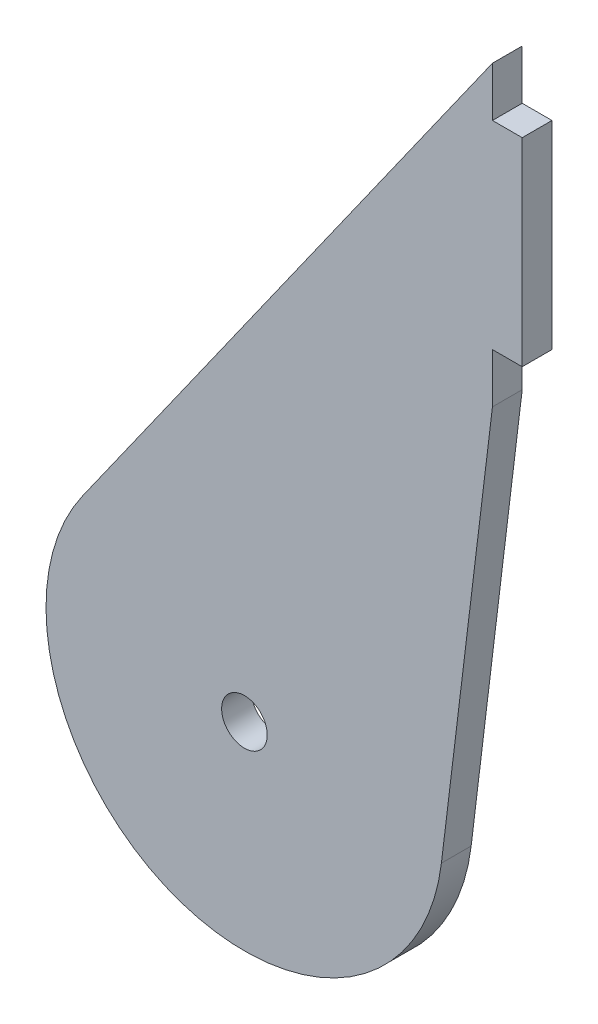
SolidWorks part; units mm, degrees
ref_plane "Front Plane" through (0, 0, 0) normal (0, 0, 1) x (1, 0, 0)
ref_plane "Top Plane" through (0, 0, 0) normal (0, 1, 0) x (1, 0, 0)
ref_plane "Right Plane" through (0, 0, 0) normal (1, 0, 0) x (0, 0, -1)
sketch "Sketch1" plane through (0, 0, 0) normal (0, 0, 1) x (1, 0, 0)
  line L0 (-16.3303, 11.5465) -> (25, 70)
  line L1 (25, 70) -> (25, 40)
  line L2 (25, 40) -> (19.8544, -2.409)
  line L3 (0, 0) -> (0, 52.3631) construction
  arc A0 (-16.3303, 11.5465) -> (19.8544, -2.409) centre (0, 0) ccw
  dimension "D6" = 20
  dimension "D7" = 25
  dimension "D8" = 70
  dimension "D9" = 30
  dimension "D10" = 6.918
extrude "Boss-Extrude1" add sketch "Sketch1" against normal blind 3
sketch "Sketch2" plane through (0, 0, 0) normal (0, 0, 1) x (1, 0, 0)
  circle A0 centre (0, 0) radius 2.3
  dimension "D1" = 4.6
extrude "Cut-Extrude1" cut sketch "Sketch2" against normal blind 10
sketch "Sketch4" plane through (25, 0, 0) normal (1, 0, 0) x (0, 0, -1)
  line L0 (0, 40) -> (0, 70) construction
  line L1 (0, 65) -> (3, 65)
  line L2 (0, 65) -> (0, 45)
  line L3 (0, 45) -> (3, 45)
  line L4 (3, 65) -> (3, 45)
  line L5 (3, 40) -> (3, 70) construction
  line L6 (3, 40) -> (0, 40) construction
  dimension "D1" = 20
  dimension "D2" = 5
extrude "Boss-Extrude3" add sketch "Sketch4" along normal blind 3
